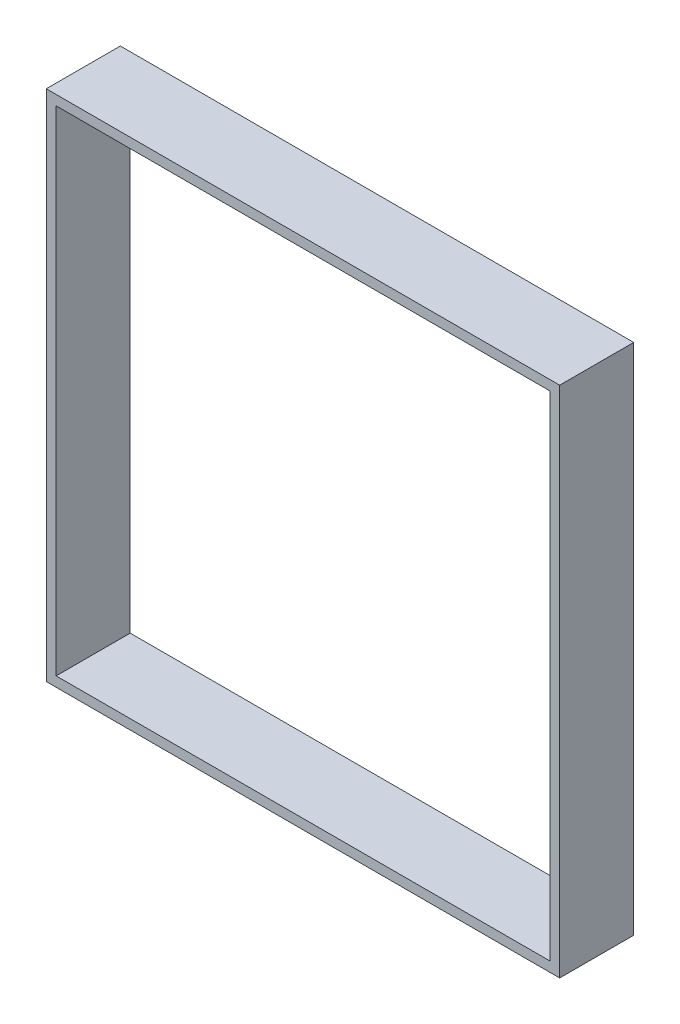
SolidWorks part; units mm, degrees
material "Q235"
ref_plane "前视基准面" through (0, 0, 0) normal (0, 0, 1) x (1, 0, 0)
ref_plane "上视基准面" through (0, 0, 0) normal (0, 1, 0) x (1, 0, 0)
ref_plane "右视基准面" through (0, 0, 0) normal (1, 0, 0) x (0, 0, -1)
sketch "草图1" plane through (0, 0, 0) normal (0, 0, 1) x (1, 0, 0)
  line L1 (100, -100) -> (-100, -100)
  line L2 (100, -100) -> (100, 100)
  line L3 (100, 100) -> (-100, 100)
  line L4 (-100, -100) -> (-100, 100)
  line L5 (100, -100) -> (-100, 100) construction
  line L6 (100, 100) -> (-100, -100) construction
  point P0 (0, 0)
  dimension "D1" = 200
  dimension "D2" = 200
extrude "拉伸-薄壁1" add sketch "草图1" along normal blind 30 thin thin type one direction wall 4
